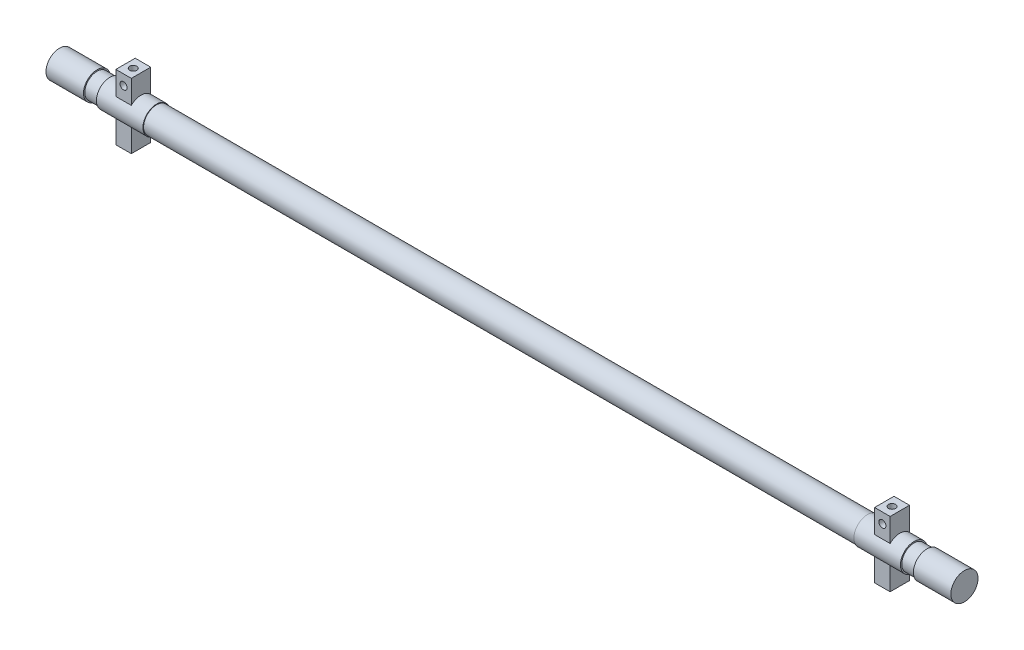
SolidWorks part; units mm, degrees
material "PC"
ref_plane "Front Plane" through (0, 0, 0) normal (0, 0, 1) x (1, 0, 0)
ref_plane "Top Plane" through (0, 0, 0) normal (0, 1, 0) x (1, 0, 0)
ref_plane "Right Plane" through (0, 0, 0) normal (1, 0, 0) x (0, 0, -1)
sketch "Sketch1" plane through (0, 0, 0) normal (0, 0, 1) x (1, 0, 0)
  line L0 (0, 0) -> (46.3477, 0) construction
  line L1 (0, 0) -> (0, 10.5)
  line L2 (0, 10.5) -> (29, 10.5)
  line L3 (29, 10.5) -> (29, 9.5)
  line L4 (29, 9.5) -> (39, 9.5)
  line L5 (39, 9.5) -> (39, 10.5)
  line L6 (39, 10.5) -> (75, 10.5)
  line L7 (75, 10.5) -> (75, 10)
  line L8 (75, 10) -> (625, 10)
  line L9 (350, 10) -> (350, 0) construction
  line L10 (700, 0) -> (0, 0)
  line L11 (625, 10.5) -> (625, 10)
  line L12 (661, 10.5) -> (625, 10.5)
  line L13 (661, 9.5) -> (661, 10.5)
  line L14 (671, 9.5) -> (661, 9.5)
  line L15 (671, 10.5) -> (671, 9.5)
  line L16 (700, 10.5) -> (671, 10.5)
  line L17 (700, 0) -> (700, 10.5)
  dimension "D1" = 20
  dimension "D2" = 21
  dimension "D3" = 75
  dimension "D4" = 700
  dimension "D5" = 1
  dimension "D6" = 29
  dimension "D7" = 10
revolve "Revolve1" add sketch "Sketch1" angle 360 about L10
sketch "Sketch2" plane through (0, 0, 0) normal (0, 0, 1) x (1, 0, 0)
  line L0 (57, 10.5) -> (57, -25) construction
  line L1 (75, 10.5) -> (39, 10.5) construction
  line L2 (0, 0) -> (57, 0) construction
  line L4 (51, 10.5) -> (63, 10.5)
  line L5 (51, 10.5) -> (51, -25)
  line L6 (51, -25) -> (63, -25)
  line L7 (63, 10.5) -> (63, -25)
  dimension "D1" = 25
  dimension "D2" = 12
  dimension "D3" = 25
extrude "Boss-Extrude1" add sketch "Sketch2" along normal mid plane 15
pattern_linear "LPattern1" count 2 spacing 587 along (1, 0, 0) of "Boss-Extrude1"
sketch "Sketch3" plane through (0, 10.5, 0) normal (0, 1, 0) x (1, 0, 0)
  line L6 (63, -7.5) -> (63, 0)
  line L7 (63, 0) -> (63, 7.5)
  line L8 (63, 7.5) -> (51, 7.5)
  line L9 (51, 7.5) -> (51, 0)
  line L10 (51, 0) -> (51, -7.5)
  line L11 (51, -7.5) -> (63, -7.5)
  line L12 (63, -7.5) -> (63, 0)
  line L13 (63, 0) -> (63, 7.5)
  line L14 (63, 7.5) -> (51, 7.5)
  line L15 (51, 7.5) -> (51, 0)
  line L16 (51, 0) -> (51, -7.5)
  line L17 (51, -7.5) -> (63, -7.5)
  line L18 (650, -7.5) -> (650, 0)
  line L19 (650, 0) -> (650, 7.5)
  line L20 (650, 7.5) -> (638, 7.5)
  line L21 (638, 7.5) -> (638, 0)
  line L22 (638, 0) -> (638, -7.5)
  line L23 (638, -7.5) -> (650, -7.5)
  line L24 (650, -7.5) -> (650, 0)
  line L25 (650, 0) -> (650, 7.5)
  line L26 (650, 7.5) -> (638, 7.5)
  line L27 (638, 7.5) -> (638, 0)
  line L28 (638, 0) -> (638, -7.5)
  line L29 (638, -7.5) -> (650, -7.5)
  dimension "D1" = 0
  dimension "D2" = 0
extrude "Boss-Extrude2" add sketch "Sketch3" along normal blind 15
hole_wizard "M5 Clearance Hole1" positions "Sketch4" profile "Sketch5" hole size "M5" standard "GB" end condition through all
sketch "Sketch4" plane through (0, 25.5, 0) normal (0, 1, 0) x (1, 0, 0)
  line L0 (51, 7.5) -> (63, -7.5) construction
  line L2 (644, 7.5) -> (644, -7.5) construction
  line L3 (650, 7.5) -> (638, 7.5) construction
  line L4 (638, -7.5) -> (650, -7.5) construction
  point P0 (57, 0)
  point P2 (644, 0)
sketch "Sketch5" plane through (57, 25.5, 0) normal (1, 0, 0) x (0, 0, 1)
  line L0 (0, 0) -> (0, 50.5)
  line L1 (0, 50.5) -> (2.75, 50.5)
  line L2 (2.75, 50.5) -> (2.75, 0)
  line L5 (2.75, 0) -> (0, 0)
  line L11 (0, -6.35) -> (0, 107.95) construction
  dimension "通孔孔直径" = 5.5
  dimension "通孔孔深度" = 50.5
hole_wizard "M5 Clearance Hole2" positions "Sketch6" profile "Sketch7" hole size "M5" standard "GB" end condition through all
sketch "Sketch6" plane through (0, 0, 7.5) normal (0, 0, 1) x (1, 0, 0)
  line L0 (57, 25.5) -> (57, 17.5) construction
  line L1 (51, 25.5) -> (63, 25.5) construction
  line L3 (644, 25.5) -> (644, 17.5) construction
  line L4 (638, 25.5) -> (650, 25.5) construction
  point P0 (57, 17.5)
  point P2 (644, 17.5)
  dimension "D1" = 8
sketch "Sketch7" plane through (57, 17.5, 7.5) normal (1, 0, 0) x (0, -1, 0)
  line L0 (0, 0) -> (0, 18)
  line L1 (0, 18) -> (2.75, 18)
  line L2 (2.75, 18) -> (2.75, 0)
  line L5 (2.75, 0) -> (0, 0)
  line L11 (0, -6.35) -> (0, 107.95) construction
  dimension "通孔孔直径" = 5.5
  dimension "通孔孔深度" = 18
